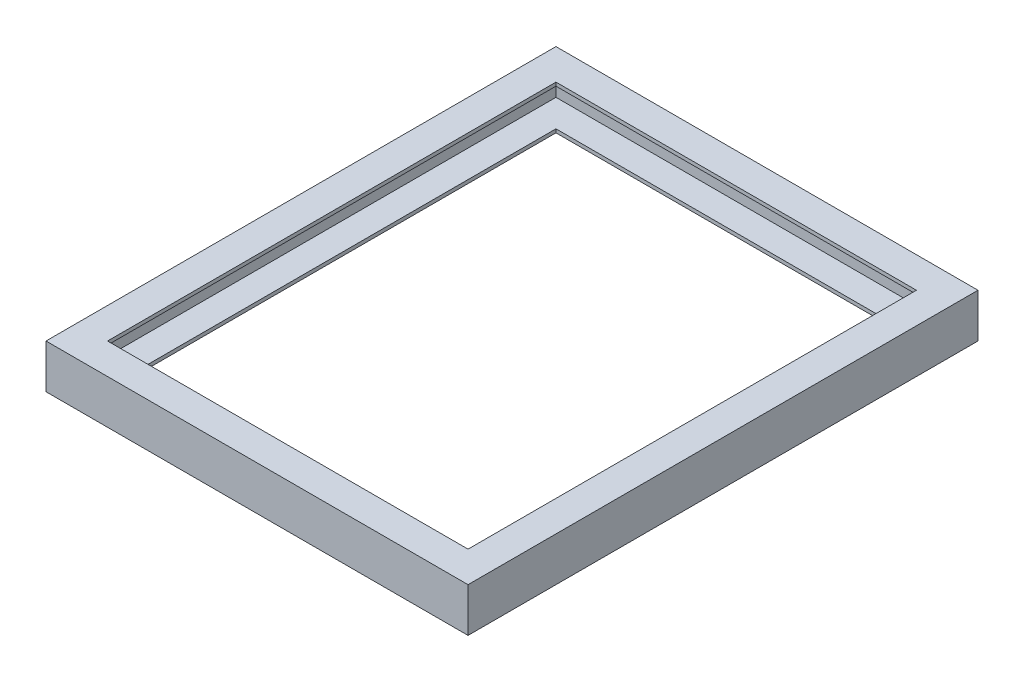
SolidWorks part; units mm, degrees
ref_plane "Front Plane" through (0, 0, 0) normal (0, 0, 1) x (1, 0, 0)
ref_plane "Top Plane" through (0, 0, 0) normal (0, 1, 0) x (1, 0, 0)
ref_plane "Right Plane" through (0, 0, 0) normal (1, 0, 0) x (0, 0, -1)
sketch "Sketch1" plane through (0, 0, 0) normal (0, 0, 1) x (1, 0, 0)
  line L0 (-10.7353, 12.7489) -> (-45.7353, 12.7489)
  line L1 (-45.7353, 12.7489) -> (-45.7353, -37.2511)
  line L2 (-45.7353, -37.2511) -> (-10.7353, -37.2511)
  line L3 (-10.7353, 8.7489) -> (-41.7353, 8.7489)
  line L4 (-41.7353, 8.7489) -> (-41.7353, -33.2511)
  line L5 (-41.7353, -33.2511) -> (-10.7353, -33.2511)
  line L6 (-10.7353, 8.7489) -> (-10.7353, 12.7489)
  line L7 (-10.7353, -33.2511) -> (-10.7353, -37.2511)
  dimension "D1" = 35
  dimension "D2" = 50
  dimension "D3" = 35
  dimension "D4" = 4
extrude "Boss-Extrude1" add sketch "Sketch1" along normal blind 580
sketch "Sketch2" plane through (-41.7353, 0, 0) normal (1, 0, 0) x (0, 0, -1)
  line L0 (-545, 12.7489) -> (-580, 12.7489)
  line L1 (-580, 12.7489) -> (0, 12.7489) construction
  line L2 (-580, 12.7489) -> (-580, -37.2511)
  line L3 (-580, -37.2511) -> (-545, -37.2511)
  line L4 (-580, -37.2511) -> (0, -37.2511) construction
  line L5 (-545, 8.7489) -> (-576, 8.7489)
  line L6 (-576, 8.7489) -> (-576, -33.2511)
  line L7 (-576, -33.2511) -> (-545, -33.2511)
  line L8 (-545, 8.7489) -> (-545, 12.7489)
  line L9 (-545, -33.2511) -> (-545, -37.2511)
  line L10 (-290, 12.7489) -> (-290, -94.646) construction
  line L11 (-35, -33.2511) -> (-35, -37.2511)
  line L12 (-35, 8.7489) -> (-35, 12.7489)
  line L13 (-4, -33.2511) -> (-35, -33.2511)
  line L14 (-4, 8.7489) -> (-4, -33.2511)
  line L15 (-35, 8.7489) -> (-4, 8.7489)
  line L16 (0, -37.2511) -> (-35, -37.2511)
  line L17 (0, 12.7489) -> (0, -37.2511)
  line L18 (-35, 12.7489) -> (0, 12.7489)
  dimension "D1" = 35
  dimension "D2" = 35
  dimension "D3" = 4
extrude "Boss-Extrude2" add sketch "Sketch2" along normal blind 472
sketch "Sketch3" plane through (0, 0, 580) normal (0, 0, 1) x (1, 0, 0)
  line L0 (399.2647, 12.7489) -> (434.2647, 12.7489)
  line L2 (430.2647, 12.7489) -> (-45.7353, 12.7489) construction
  line L3 (434.2647, 12.7489) -> (434.2647, -37.2511)
  line L5 (434.2647, -37.2511) -> (399.2647, -37.2511)
  line L6 (-45.7353, -37.2511) -> (430.2647, -37.2511) construction
  line L7 (399.2647, 8.7489) -> (430.2647, 8.7489)
  line L8 (430.2647, 8.7489) -> (430.2647, -33.2511)
  line L9 (430.2647, -33.2511) -> (399.2647, -33.2511)
  line L10 (430.2647, 12.7489) -> (430.2647, -37.2511) construction
  line L11 (399.2647, 8.7489) -> (399.2647, 12.7489)
  line L12 (399.2647, -33.2511) -> (399.2647, -37.2511)
  dimension "D1" = 35
  dimension "D2" = 35
  dimension "D3" = 50
  dimension "D5" = 0
  dimension "D4" = 4
extrude "Boss-Extrude3" add sketch "Sketch3" against normal blind 580
